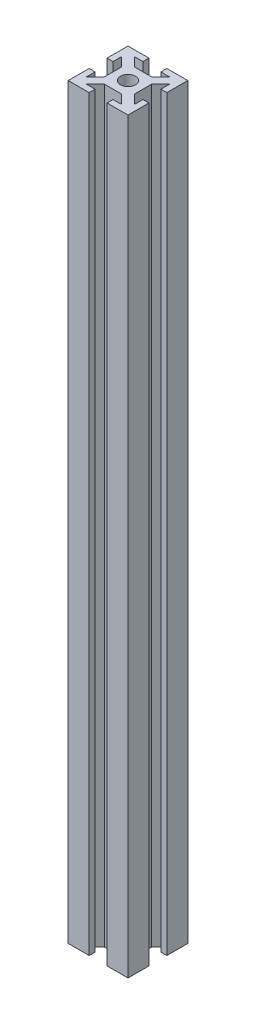
from build123d import *

# Parameters (mm, degrees)
SKETCH1_R           = 5
BOSS_EXTRUDE1_DEPTH = 500


with BuildPart() as part:
    # Sketch1 → Boss-Extrude1 (new body)
    with BuildSketch(Plane(origin=(0, 0, 0), x_dir=(1, 0, 0), z_dir=(0, 1, 0))):
        Polygon((-6, 20), (-6, 16), (-11.757359313, 16), (-5.757359313, 10), (5.757359313, 10), (11.757359313, 16), (6, 16), (6, 20), (20, 20), (20, 6), (16, 6), (16, 11.757359313), (10, 5.757359313), (10, -5.757359313), (16, -11.757359313), (16, -6), (20, -6), (20, -20), (6, -20), (6, -16), (11.757359313, -16), (5.757359313, -10), (-5.757359313, -10), (-11.757359313, -16), (-6, -16), (-6, -20), (-20, -20), (-20, -6), (-16, -6), (-16, -11.757359313), (-10, -5.757359313), (-10, 5.757359313), (-16, 11.757359313), (-16, 6), (-20, 6), (-20, 20), align=None)
        with Locations(Location((0, 0, 0), (0, 0, 270))):
            Circle(SKETCH1_R, mode=Mode.SUBTRACT)
    extrude(amount=BOSS_EXTRUDE1_DEPTH)


solid = part.part
